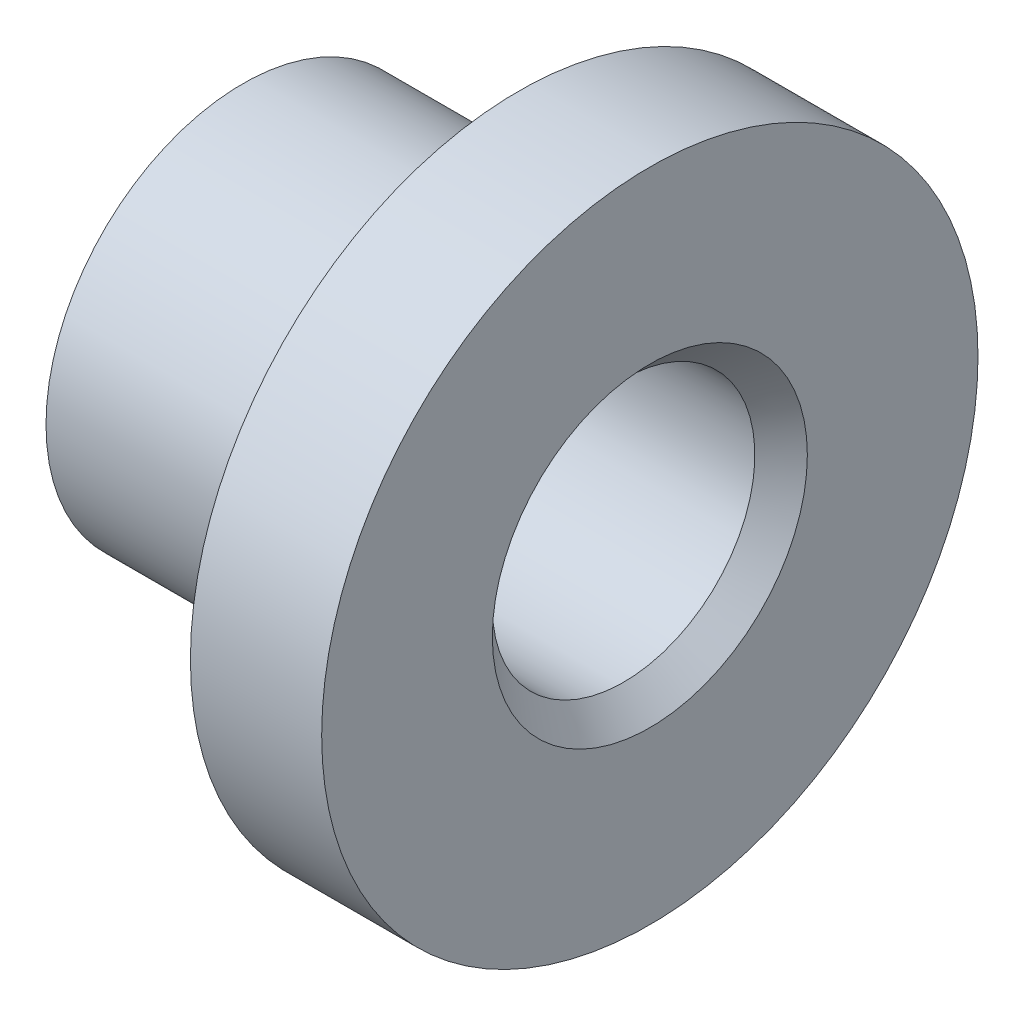
SolidWorks part; units mm, degrees
ref_plane "Front" through (0, 0, 0) normal (0, 0, 1) x (1, 0, 0)
ref_plane "Top" through (0, 0, 0) normal (0, 1, 0) x (1, 0, 0)
ref_plane "Right" through (0, 0, 0) normal (1, 0, 0) x (0, 0, -1)
sketch "Sketch1" plane through (0, 0, 0) normal (0, 0, 1) x (1, 0, 0)
  line L0 (-31.6626, 0) -> (37.2861, 0) construction
  line L1 (-20.7824, 10) -> (10.2176, 10)
  line L2 (10.2176, 10) -> (10.2176, 25)
  line L3 (10.2176, 25) -> (0.2176, 25)
  line L4 (0.2176, 25) -> (0.2176, 15)
  line L5 (0.2176, 15) -> (-20.7824, 15)
  line L6 (-20.7824, 15) -> (-20.7824, 10)
  dimension "D1" = 25
  dimension "D2" = 10
  dimension "D3" = 10
  dimension "D4" = 21
  dimension "D5" = 15
revolve "Revolve1" add sketch "Sketch1" angle 360 about L0
chamfer "Chamfer1" distance 2 angle 45 1 edges at (10.2176, 0, 10)
equation "\"零件重量\"= IIF ( \"SW-质量\" > 100 , int ( \"SW-质量\" ) , \"SW-质量\" )"
